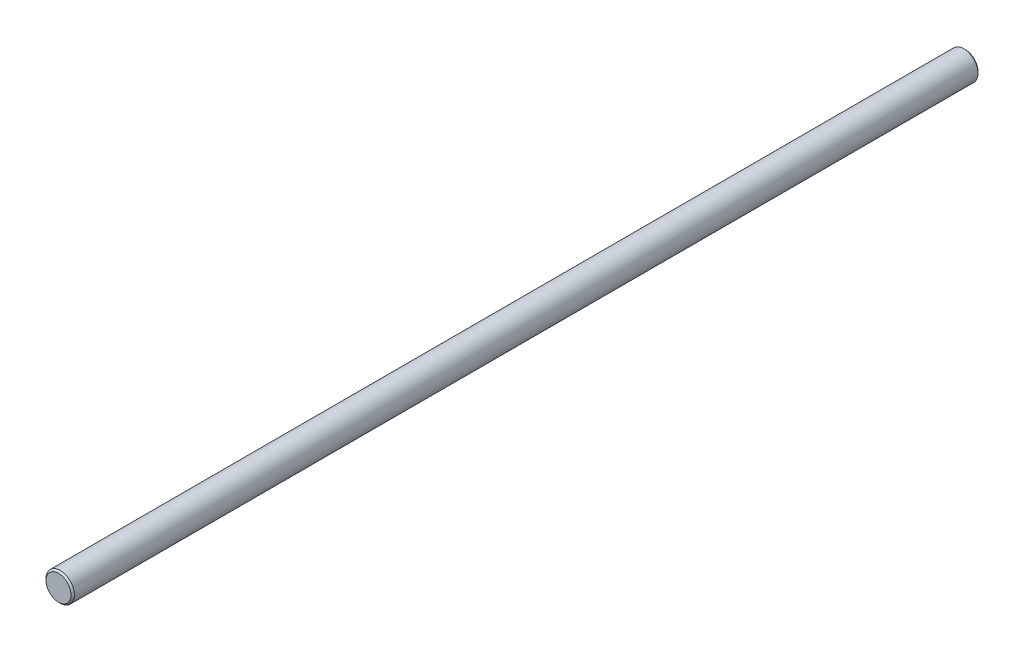
SolidWorks part; units mm, degrees
ref_plane "Front Plane" through (0, 0, 0) normal (0, 0, 1) x (1, 0, 0)
ref_plane "Top Plane" through (0, 0, 0) normal (0, 1, 0) x (1, 0, 0)
ref_plane "Right Plane" through (0, 0, 0) normal (1, 0, 0) x (0, 0, -1)
sketch "Sketch1" plane through (0, 0, 0) normal (0, 0, 1) x (1, 0, 0)
  circle A0 centre (0, 0) radius 4.25
  dimension "D1" = 8.5
extrude "Boss-Extrude1" add sketch "Sketch1" along normal blind 271.5
chamfer "Chamfer1" distance 0.5 angle 45 2 edges at (4.25, 0, 271.5) (4.25, 0, 0)
